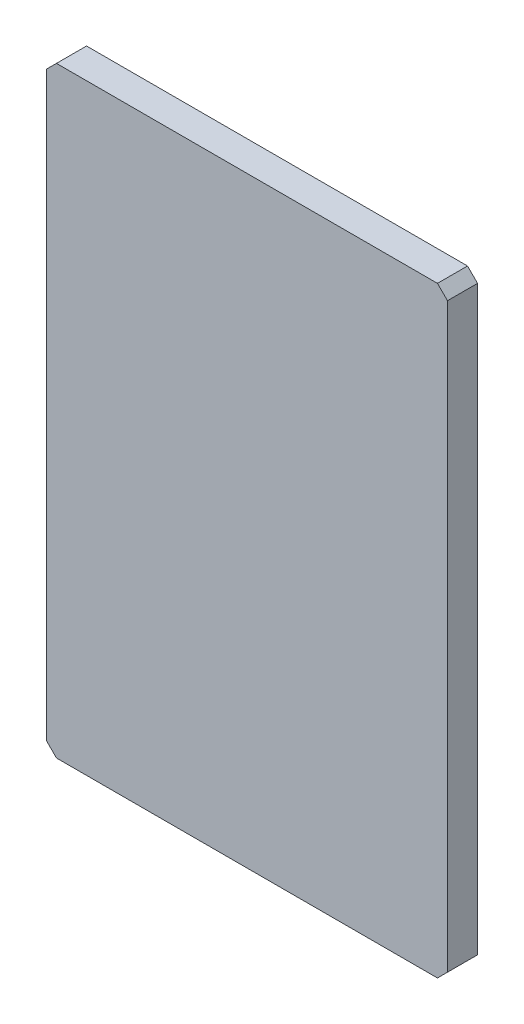
from build123d import *

# Parameters (mm, degrees)
SKETCH_1_W      = 200
SKETCH_1_H      = 300
EXTRUDE_1_DEPTH = 7.5
CHAMFER_1_SIZE  = 5


with BuildPart() as part:
    # 草图1 → 凸台-拉伸1 (new, symmetric)
    with BuildSketch(Plane.XY):
        Rectangle(SKETCH_1_W, SKETCH_1_H)
    extrude(amount=EXTRUDE_1_DEPTH, both=True)

    # 倒角1
    chamfer_1_edges = [part.edges().sort_by_distance(p)[0] for p in [
        (100, -150, 0),
        (-100, -150, 0),
        (-100, 150, 0),
        (100, 150, 0),
    ]]
    chamfer(chamfer_1_edges, length=CHAMFER_1_SIZE)


solid = part.part
